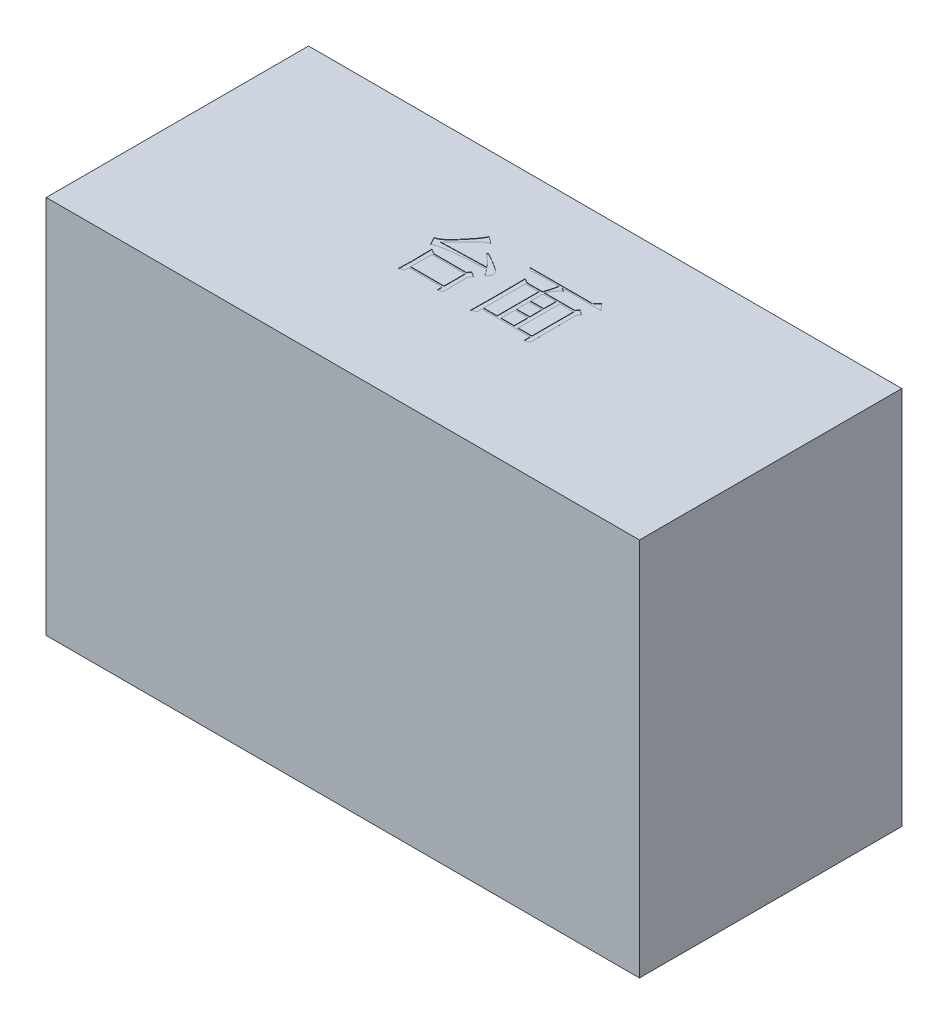
from build123d import *

# Parameters (mm, degrees)
SKETCH_1_W          = 1470
SKETCH_1_H          = 940
EXTRUDE_1_DEPTH     = 650
SKETCH_2_W          = 82.551690925
SKETCH_2_H          = 52.062714041
SKETCH_2_W_2        = 32.403467465
SKETCH_2_H_2        = 33.775042808
SKETCH_2_W_3        = 33.174978596
SKETCH_2_H_3        = 103.268193493
SKETCH_2_W_4        = 33.946489726
SKETCH_2_H_4        = 30.117508562
CUT_EXTRUDE_1_DEPTH = 1


with BuildPart() as part:
    # 草图1 → 凸台-拉伸1 (new body)
    with BuildSketch(Plane.XY):
        Rectangle(SKETCH_1_W, SKETCH_1_H)
    extrude(amount=EXTRUDE_1_DEPTH)

    # 草图2 → 切除-拉伸1 (cut)
    # profile 1 of 3: a face of its own
    with BuildSketch(Plane(origin=(0, 470, 0), x_dir=(1, 0, 0), z_dir=(0, 1, 0))):
        with BuildLine():
            Line((-150.986660578, -256.848387178), (-39.117546708, -253.762342658))
            add(Edge.make_bspline(
                [(-39.117546708, -253.762342658), (-39.880022564, -252.811744564), (-41.499389472, -250.792838548), (-44.2612406, -247.755235558), (-47.425086622, -244.459461375), (-50.972852336, -240.899252546), (-54.969668459, -237.132882567), (-59.332720324, -233.103001721), (-64.1176634, -228.838443301), (-67.468857374, -225.945128673), (-69.206480783, -224.444919713)],
                knots=[0, 0, 0, 0, 0.695110772, 1.476295114, 2.341084901, 3.301725276, 4.343406775, 5.4740605, 6.690278259, 8, 8, 8, 8], degree=3))
            Line((-69.206480783, -224.444919713), (-66.891947393, -222.130386322))
            add(Edge.make_bspline(
                [(-66.891947393, -222.130386322), (-64.547569523, -223.43300718), (-60.033447357, -225.941216187), (-53.570239406, -229.580115106), (-47.68039296, -232.965489978), (-42.385188654, -236.091803599), (-37.665690899, -238.972743769), (-33.480812748, -241.498867528), (-29.940632546, -243.874321965), (-26.885349292, -245.941477825), (-24.266168738, -247.864044928), (-22.100543663, -249.829740826), (-20.20893879, -251.742556628), (-18.666894954, -253.670671714), (-17.454201979, -255.611187476), (-16.636383887, -257.564489809), (-16.069446795, -259.512385826), (-16.004449158, -260.825967458), (-15.972212804, -261.477453959)],
                knots=[0, 0, 0, 0, 1.942818502, 3.740915738, 5.372963559, 6.863959824, 8.195192806, 9.37858452, 10.404314035, 11.282759543, 12.051398879, 12.755043522, 13.399131945, 13.998263769, 14.540238823, 15.050311193, 15.528990492, 16, 16, 16, 16], degree=3))
            add(Edge.make_bspline(
                [(-15.972212804, -261.477453959), (-16.008170239, -261.926922674), (-16.091916424, -262.973751781), (-16.560461021, -264.716244258), (-17.333219173, -266.826355635), (-18.250562762, -269.173608987), (-19.270568705, -271.393311343), (-20.25256785, -273.081945244), (-21.125971852, -274.265880541), (-21.854265464, -274.499933633), (-22.144301845, -274.593143171)],
                knots=[0, 0, 0, 0, 0.723904269, 1.68599957, 2.887289168, 4.337768568, 5.74231969, 6.792987712, 7.519318212, 8, 8, 8, 8], degree=3))
            add(Edge.make_bspline(
                [(-22.144301845, -274.593143171), (-22.523744704, -274.553315178), (-23.289219503, -274.472967572), (-24.347580784, -273.82646771), (-25.266427162, -272.815465308), (-25.74339744, -271.966911774), (-26.001857496, -271.507098651)],
                knots=[0, 0, 0, 0, 0.871549862, 1.758234318, 2.785234828, 4, 4, 4, 4], degree=3))
            add(Edge.make_bspline(
                [(-26.001857496, -271.507098651), (-27.529736342, -269.248543868), (-30.528811326, -264.815224323), (-33.70292815, -260.505529901), (-35.259991057, -258.391409439)],
                knots=[0, 0, 0, 0, 1.018900064, 2, 2, 2, 2], degree=3))
            add(Edge.make_bspline(
                [(-35.259991057, -258.391409439), (-37.99388467, -258.459551519), (-43.539109983, -258.597765819), (-51.968027384, -258.959217828), (-60.618144289, -259.373940526), (-69.47547602, -259.928619508), (-78.552611055, -260.560110294), (-87.850798883, -261.263749745), (-97.364930129, -262.101871201), (-105.373789255, -262.860333809), (-111.749432485, -263.479248117), (-116.336106143, -264.042839339), (-120.722787544, -264.565392698), (-124.884002526, -265.170089335), (-128.824504806, -265.807374972), (-132.5556212, -266.4186387), (-136.058720067, -267.110840281), (-139.356115984, -267.820947237), (-142.429008822, -268.571313856), (-145.298563064, -269.29276348), (-147.932553086, -270.105596113), (-150.356161352, -270.925507846), (-152.576091253, -271.776298273), (-154.557866405, -272.696922868), (-156.3494304, -273.591870467), (-157.420724483, -274.270411036), (-157.930260749, -274.593143171)],
                knots=[0, 0, 0, 0, 1.58148585, 3.207767604, 4.878815534, 6.589581641, 8.339901368, 10.140867898, 11.982062348, 13.863148664, 14.793262735, 15.686247323, 16.535485185, 17.347968149, 18.117707415, 18.843963216, 19.534256627, 20.182502326, 20.794390892, 21.363530801, 21.893241407, 22.387943635, 22.843134266, 23.267091727, 23.651409122, 24, 24, 24, 24], degree=3))
            Line((-157.930260749, -274.593143171), (-168.731416571, -255.305364918))
            add(Edge.make_bspline(
                [(-168.731416571, -255.305364918), (-168.137959074, -255.213936591), (-166.897208498, -255.022786003), (-165.021215999, -254.451565233), (-163.024673291, -253.712321561), (-160.951232194, -252.697758767), (-158.77493337, -251.467770352), (-156.524545816, -249.988981232), (-154.13620822, -248.344887947), (-151.669288965, -246.39095672), (-149.0037747, -244.181111607), (-146.180686108, -241.5683682), (-143.161922884, -238.546286367), (-139.876866541, -235.190911988), (-136.386185446, -231.440233153), (-132.712247829, -227.286014447), (-128.789268839, -222.768358948), (-124.743675962, -217.97272562), (-120.773871695, -213.103035552), (-117.040835679, -208.398548034), (-113.714843871, -203.916388063), (-110.713953148, -199.71451065), (-108.121104022, -195.73741191), (-105.851152448, -192.032831407), (-103.946923611, -188.573480952), (-102.885066126, -186.312865663), (-102.381459379, -185.240724507)],
                knots=[0, 0, 0, 0, 0.438738821, 0.917277897, 1.431042448, 1.995118532, 2.603539808, 3.258718438, 3.964239441, 4.723837876, 5.559749051, 6.49668025, 7.536257587, 8.684309132, 9.931590992, 11.283847934, 12.740947079, 14.308413863, 15.873261316, 17.336876234, 18.701142671, 19.955798073, 21.113388014, 22.173313975, 23.133658312, 24, 24, 24, 24], degree=3))
            Line((-102.381459379, -185.240724507), (-84.636703386, -198.327839233))
            add(Edge.make_bspline(
                [(-84.636703386, -198.327839233), (-86.011497365, -198.638377891), (-88.741634574, -199.255061668), (-92.601745081, -200.919442138), (-96.177521062, -203.163143828), (-98.246936048, -205.074535153), (-99.295414859, -206.042950534)],
                knots=[0, 0, 0, 0, 1.003882844, 1.993562635, 2.983429097, 4, 4, 4, 4], degree=3))
            add(Edge.make_bspline(
                [(-99.295414859, -206.042950534), (-99.640936575, -206.37368019), (-100.429292886, -207.128286336), (-101.693312474, -208.474359202), (-103.350033963, -210.007853343), (-105.21662639, -211.923113501), (-107.415591454, -214.076990334), (-109.918071847, -216.517729653), (-112.706230692, -219.254029191), (-115.804347453, -222.280210087), (-119.154760662, -225.635751995), (-122.854767991, -229.2121493), (-126.80309895, -233.131753907), (-131.073392704, -237.300230496), (-135.63335624, -241.779374798), (-140.482977619, -246.54027968), (-145.626697812, -251.607349522), (-149.16628379, -255.068400319), (-150.986660578, -256.848387178)],
                knots=[0, 0, 0, 0, 0.316715718, 0.722631381, 1.22226937, 1.811034564, 2.493481524, 3.260712275, 4.126064678, 5.080619631, 6.12880958, 7.266275595, 8.488441964, 9.813231229, 11.218302795, 12.721497735, 14.313896185, 16, 16, 16, 16], degree=3))
        make_face()
    # profile 2 of 3: a face of its own
    with BuildSketch(Plane(origin=(0, 470, 0), x_dir=(1, 0, 0), z_dir=(0, 1, 0))):
        with BuildLine():
            add(Edge.make_bspline(
                [(-146.357593797, -366.288669713), (-146.301037075, -364.878982692), (-146.184871399, -361.983531183), (-145.994530042, -357.527052808), (-145.904031313, -352.839489356), (-145.776017583, -347.91569771), (-145.69282615, -342.762543502), (-145.647105565, -337.371269895), (-145.56988038, -331.751824387), (-145.591021773, -324.036435844), (-145.622426923, -314.492232328), (-145.771942175, -303.376499559), (-145.979347222, -292.812048315), (-146.233853149, -285.955987147), (-146.357593797, -282.622573822)],
                knots=[0, 0, 0, 0, 0.606909075, 1.246571595, 1.918740328, 2.623678739, 3.365404803, 4.135754193, 4.942977934, 5.782939047, 7.454686618, 9.048695707, 10.565077409, 12, 12, 12, 12], degree=3))
            Line((-146.357593797, -282.622573822), (-134.013415715, -290.337685123))
            Line((-134.013415715, -290.337685123), (-53.77625818, -290.337685123))
            Line((-53.77625818, -290.337685123), (-48.375680269, -282.622573822))
            Line((-48.375680269, -282.622573822), (-34.488479927, -291.109196254))
            Line((-34.488479927, -291.109196254), (-41.432080098, -297.39558324))
            Line((-41.432080098, -297.39558324), (-41.432080098, -337.342715089))
            add(Edge.make_bspline(
                [(-41.432080098, -337.342715089), (-41.418067905, -338.876306289), (-41.388298079, -342.134521557), (-41.232409185, -347.316209576), (-41.013360182, -353.089522849), (-40.782002112, -357.135650816), (-40.660568968, -359.259346082)],
                knots=[0, 0, 0, 0, 0.839084402, 1.782689943, 2.836198234, 4, 4, 4, 4], degree=3))
            Line((-40.660568968, -359.259346082), (-52.23323592, -364.745647452))
            Line((-52.23323592, -364.745647452), (-52.23323592, -351.658532726))
            Line((-52.23323592, -351.658532726), (-134.784926845, -351.658532726))
            Line((-134.784926845, -351.658532726), (-134.784926845, -360.888091802))
            Line((-134.784926845, -360.888091802), (-146.357593797, -366.288669713))
        make_face()
        with Locations((-93.509081382, -320.998108925)):
            Rectangle(SKETCH_2_W, SKETCH_2_H, mode=Mode.SUBTRACT)
    # profile 3 of 3: a face of its own
    with BuildSketch(Plane(origin=(0, 470, 0), x_dir=(1, 0, 0), z_dir=(0, 1, 0))):
        with BuildLine():
            add(Edge.make_bspline(
                [(82.009700724, -237.303438548), (82.992665776, -234.512867527), (84.914346213, -229.057347282), (87.216375779, -220.905868769), (89.165349818, -213.063726453), (90.059337756, -207.887383171), (90.496323155, -205.357162863)],
                knots=[0, 0, 0, 0, 1.072281711, 2.09629303, 3.069459313, 4, 4, 4, 4], degree=3))
            Line((90.496323155, -205.357162863), (41.119610826, -205.357162863))
            add(Edge.make_bspline(
                [(41.119610826, -205.357162863), (39.25186169, -205.382910535), (35.644459622, -205.432640022), (30.422521922, -205.860192402), (25.588445461, -206.581712608), (22.532375579, -207.317351954), (21.060321443, -207.671696254)],
                knots=[0, 0, 0, 0, 1.106811247, 2.137713842, 3.102970106, 4, 4, 4, 4], degree=3))
            Line((21.060321443, -207.671696254), (14.116721272, -200.728096082))
            Line((14.116721272, -200.728096082), (168.418947299, -200.728096082))
            Line((168.418947299, -200.728096082), (180.763125381, -188.898258754))
            Line((180.763125381, -188.898258754), (194.650325724, -205.357162863))
            Line((194.650325724, -205.357162863), (98.211434457, -205.357162863))
            Line((98.211434457, -205.357162863), (109.784101409, -211.300656014))
            Line((109.784101409, -211.300656014), (102.068990107, -213.529465945))
            add(Edge.make_bspline(
                [(102.068990107, -213.529465945), (100.581994075, -215.598394294), (97.681126945, -219.634508789), (93.614595512, -225.664968228), (89.948675288, -231.519177202), (87.722033314, -235.41036691), (86.638767504, -237.303438548)],
                knots=[0, 0, 0, 0, 1.078061173, 2.103107307, 3.07715788, 4, 4, 4, 4], degree=3))
            Line((86.638767504, -237.303438548), (162.246858258, -237.303438548))
            Line((162.246858258, -237.303438548), (167.647436169, -229.588327247))
            Line((167.647436169, -229.588327247), (179.991614251, -238.846460808))
            Line((179.991614251, -238.846460808), (174.59103634, -244.247038719))
            add(Edge.make_bspline(
                [(174.59103634, -244.247038719), (174.585484175, -249.923846547), (174.574622021, -261.029849642), (174.652232552, -277.326761901), (174.697296451, -292.890411021), (174.781123877, -307.730168903), (174.908735144, -321.845777706), (174.999175719, -335.247685699), (175.189003705, -347.924841127), (175.305874354, -356.135199555), (175.36254747, -360.116580671)],
                knots=[0, 0, 0, 0, 1.175793828, 2.300301559, 3.375489397, 4.399394081, 5.373993396, 6.299274203, 7.175281124, 8, 8, 8, 8], degree=3))
            Line((175.36254747, -360.116580671), (163.789880518, -365.517158582))
            Line((163.789880518, -365.517158582), (163.789880518, -349.829765603))
            Line((163.789880518, -349.829765603), (44.205655347, -349.829765603))
            Line((44.205655347, -349.829765603), (44.205655347, -360.802368343))
            Line((44.205655347, -360.802368343), (32.632988395, -366.288669713))
            add(Edge.make_bspline(
                [(32.632988395, -366.288669713), (32.689695569, -363.955083019), (32.806811092, -359.13560068), (32.997017902, -351.66880377), (33.086928981, -343.733806663), (33.214615702, -335.333225276), (33.298499829, -326.465480999), (33.34288309, -317.121493016), (33.423406578, -307.301508782), (33.394790284, -297.18603747), (33.423481061, -287.118187525), (33.343407345, -277.450599432), (33.298592871, -268.344731666), (33.215580434, -259.810335618), (33.087968916, -251.838386096), (32.997628393, -244.427193315), (32.809830298, -237.589017975), (32.690111164, -233.21727991), (32.632988395, -231.131349507)],
                knots=[0, 0, 0, 0, 0.828918971, 1.711939972, 2.652324654, 3.646821298, 4.695392265, 5.801434409, 6.964975116, 8.182613417, 9.39348706, 10.540116414, 11.615718185, 12.627085344, 13.570852006, 14.446979584, 15.258992086, 16, 16, 16, 16], degree=3))
            Line((32.632988395, -231.131349507), (44.205655347, -237.303438548))
            Line((44.205655347, -237.303438548), (82.009700724, -237.303438548))
        make_face()
        with Locations((103.612012368, -328.313177418)):
            Rectangle(SKETCH_2_W_2, SKETCH_2_H_2, mode=Mode.SUBTRACT)
        with Locations((60.793144645, -293.566602076)):
            Rectangle(SKETCH_2_W_3, SKETCH_2_H_3, mode=Mode.SUBTRACT)
        with Locations((146.816635655, -293.566602076)):
            Rectangle(SKETCH_2_W_4, SKETCH_2_H_3, mode=Mode.SUBTRACT)
        with Locations((103.612012368, -256.99125961)):
            Rectangle(SKETCH_2_W_2, SKETCH_2_H_4, mode=Mode.SUBTRACT)
        with Locations((103.612012368, -291.737834952)):
            Rectangle(SKETCH_2_W_2, SKETCH_2_H_4, mode=Mode.SUBTRACT)
    extrude(amount=-CUT_EXTRUDE_1_DEPTH, mode=Mode.SUBTRACT)


solid = part.part
